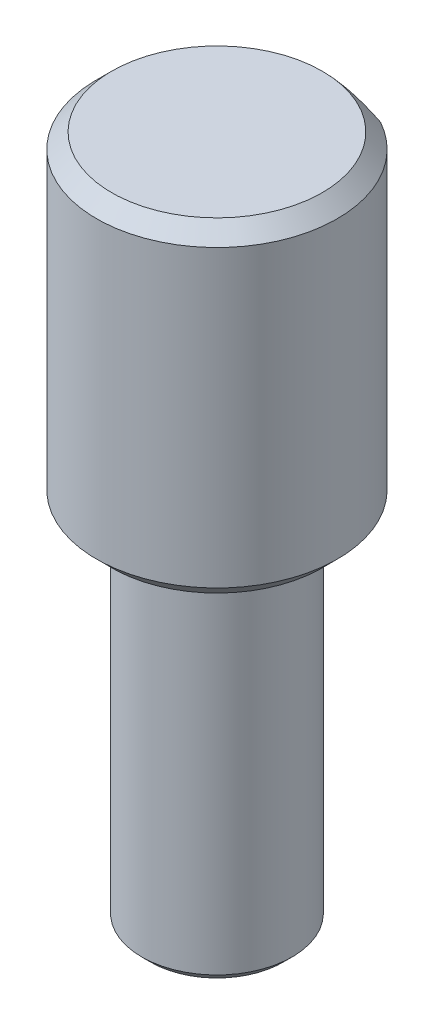
SolidWorks part; units mm, degrees
ref_plane "Front Plane" through (0, 0, 0) normal (0, 0, 1) x (1, 0, 0)
ref_plane "Top Plane" through (0, 0, 0) normal (0, 1, 0) x (1, 0, 0)
ref_plane "Right Plane" through (0, 0, 0) normal (1, 0, 0) x (0, 0, -1)
sketch "Sketch1" plane through (0, 0, 0) normal (0, 1, 0) x (1, 0, 0)
  circle A0 centre (0, 0) radius 2.5
  dimension "D1" = 5
extrude "Boss-Extrude1" add sketch "Sketch1" along normal blind 12
sketch "Sketch2" plane through (0, 12, 0) normal (0, 1, 0) x (1, 0, 0)
  circle A0 centre (0, 0) radius 4
  dimension "D1" = 8
extrude "Boss-Extrude2" add sketch "Sketch2" along normal blind 10.8
chamfer "Chamfer1" distance 0.5 angle 45 2 edges at (0, 22.8, 4) (0, 12, 4)
chamfer "Chamfer2" distance 0.3 angle 45 1 edges at (0, 0, 2.5)
sketch "Sketch3" plane through (0, 22.8, 0) normal (0, 1, 0) x (1, 0, 0)
  line L0 (0, 0) -> (0, -50000) construction
  line L2 (-4.0002, 4.5) -> (4.0002, 4.5)
  line L3 (-4.0002, 4.5) -> (-4.0002, 3.5)
  line L4 (-4.0002, 3.5) -> (4.0002, 3.5)
  line L5 (4.0002, 4.5) -> (4.0002, 3.5)
  line L6 (-4.0002, 4.5) -> (4.0002, 3.5) construction
  line L7 (-4.0002, 3.5) -> (4.0002, 4.5) construction
  circle A0 centre (0, 0) radius 4 construction
  point P3 (0, 4)
  dimension "D1" = 3.5
extrude "Cut-Extrude1" cut sketch "Sketch3" against normal blind 12
hole_wizard "M3 Tapped Hole1" positions "Sketch5" profile "Sketch4" tap size "M3" standard "Gb"
sketch "Sketch5" plane through (0, 0, 0) normal (0, -1, 0) x (-1, 0, 0)
  point P0 (0, 0)
sketch "Sketch4" plane through (0, 0, 0) normal (1, 0, 0) x (0, 0, -1)
  line L0 (0, 0) -> (0, 8.2511)
  line L1 (0, 8.2511) -> (1.25, 7.5)
  line L2 (1.25, 7.5) -> (1.25, 0)
  line L5 (1.25, 0) -> (0, 0)
  line L10 (0, 8.2511) -> (-1.25, 7.5) construction
  line L11 (0, -6.35) -> (0, 107.95) construction
  dimension "螺纹孔钻头直径" = 2.5
  dimension "螺纹孔钻头深度" = 7.5
  dimension "导头角度" = 118
cosmetic thread "Hole Thread1" parameters "D1"=6, "D2"=3
